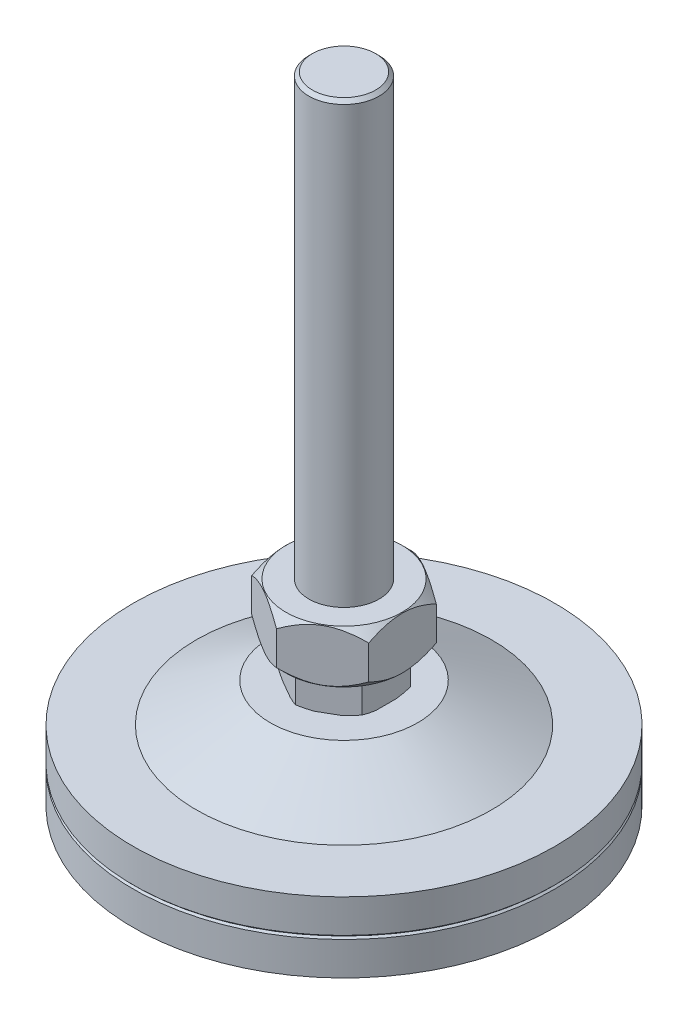
SolidWorks part; units mm, degrees
material "普通碳钢"
ref_plane "Front Plane" through (0, 0, 0) normal (0, 0, 1) x (1, 0, 0)
ref_plane "Top Plane" through (0, 0, 0) normal (0, 1, 0) x (1, 0, 0)
ref_plane "Right Plane" through (0, 0, 0) normal (1, 0, 0) x (0, 0, -1)
sketch "Sketch1" plane through (0, 0, 0) normal (0, 0, 1) x (1, 0, 0)
  line L0 (35, 0) -> (60, 0)
  line L1 (60, 0) -> (60, 9.5)
  line L2 (60, 20) -> (42, 20)
  line L3 (42, 20) -> (21, 31)
  line L4 (21, 31) -> (10, 31)
  line L5 (10, 31) -> (10, 181)
  line L6 (10, 181) -> (0, 181)
  line L7 (0, 181) -> (0, 15)
  line L8 (60, 10) -> (59.189, 10) construction
  line L9 (60, 10.5) -> (59.5, 10)
  line L10 (59.5, 10) -> (60, 9.5)
  line L11 (0, 15) -> (14, 15)
  line L12 (14, 15) -> (35, 0)
  line L13 (55, 0) -> (-55, 0) construction
  line L14 (60, 10.5) -> (60, 20)
  line L15 (0, 15) -> (0, 0) construction
  point P0 (5, 181)
  dimension "D1" = 20
  dimension "D2" = 181
  dimension "D3" = 10
  dimension "D4" = 11
  dimension "D5" = 31
  dimension "D6" = 18
  dimension "D7" = 60
  dimension "D8" = 10
  dimension "D9" = 0.5
  dimension "D10" = 1
  dimension "D11" = 0.5
  dimension "D12" = 15
  dimension "D13" = 25
  dimension "D14" = 14
  dimension "D15" = 45
revolve "Revolve1" add sketch "Sketch1" angle 360 about L7
cosmetic thread "Cosmetic Thread1" parameters "D2"=19
sketch "Sketch2" plane through (0, 31, 0) normal (0, 1, 0) x (1, 0, 0)
  line L1 (12, 6.9282) -> (0, 13.8564)
  line L2 (0, 13.8564) -> (-12, 6.9282)
  line L3 (-12, 6.9282) -> (-12, -6.9282)
  line L4 (-12, -6.9282) -> (0, -13.8564)
  line L5 (0, -13.8564) -> (12, -6.9282)
  line L6 (12, -6.9282) -> (12, 6.9282)
  circle A0 centre (0, 0) radius 12 construction
  dimension "D1" = 24
extrude "Boss-Extrude1" add sketch "Sketch2" along normal blind 9
sketch "Sketch3" plane through (0, 0, 0) normal (1, 0, 0) x (0, 0, -1)
  line L0 (12.3564, 31) -> (13.8564, 31.866)
  line L1 (6.9282, 31) -> (13.8564, 31) construction
  line L2 (13.8564, 40) -> (13.8564, 31) construction
  line L3 (13.8564, 31.866) -> (13.8564, 31)
  line L4 (13.8564, 39.4226) -> (12.8564, 40)
  line L5 (6.9282, 40) -> (13.8564, 40) construction
  line L6 (12.8564, 40) -> (13.8564, 40)
  line L7 (13.8564, 40) -> (13.8564, 39.4226)
  line L8 (21, 31) -> (-21, 31) construction
  line L9 (13.8564, 31) -> (12.3564, 31)
  dimension "D1" = 30
  dimension "D2" = 1.5
  dimension "D3" = 30
  dimension "D4" = 1
revolve "Cut-Revolve1" cut sketch "Sketch3" angle 360 about axis through (0, 181, 0) along (0, 1, 0)
ref_plane "Plane1" through (0, 41, 0) normal (0, 1, 0) x (-1, 0, 0)
sketch "Sketch5" plane through (0, 41, 0) normal (0, 1, 0) x (-1, 0, 0)
  line L1 (0, 19.2258) -> (-16.65, 9.6129)
  line L2 (-16.65, 9.6129) -> (-16.65, -9.6129)
  line L3 (-16.65, -9.6129) -> (0, -19.2258)
  line L4 (0, -19.2258) -> (16.65, -9.6129)
  line L5 (16.65, -9.6129) -> (16.65, 9.6129)
  line L6 (16.65, 9.6129) -> (0, 19.2258)
  circle A0 centre (0, 0) radius 16.65 construction
  circle A1 centre (0, 0) radius 10
  dimension "D1" = 33.3
  dimension "D2" = 20
extrude "Boss-Extrude2" add sketch "Sketch5" along normal blind 15
sketch "Sketch7" plane through (0, 0, 0) normal (1, 0, 0) x (0, 0, -1)
  line L0 (16.5258, 56) -> (19.2258, 53.3)
  line L1 (9.6129, 56) -> (19.2258, 56) construction
  line L2 (19.2258, 56) -> (19.2258, 41) construction
  line L3 (19.2258, 53.3) -> (19.2258, 56)
  line L4 (19.2258, 56) -> (16.5258, 56)
  line L5 (16.5258, 41) -> (19.2258, 43.7)
  line L6 (23.1, 41) -> (-23.1, 41) construction
  line L7 (19.2258, 43.7) -> (19.2258, 41)
  line L8 (19.2258, 41) -> (16.5258, 41)
  dimension "D1" = 45
  dimension "D2" = 2.7
  dimension "D3" = 2.7
  dimension "D4" = 45
revolve "Cut-Revolve3" cut sketch "Sketch7" angle 360 about axis through (0, 181, 0) along (0, 1, 0)
chamfer "Chamfer1" distance 1 angle 45 1 edges at (-10, 181, 0)
